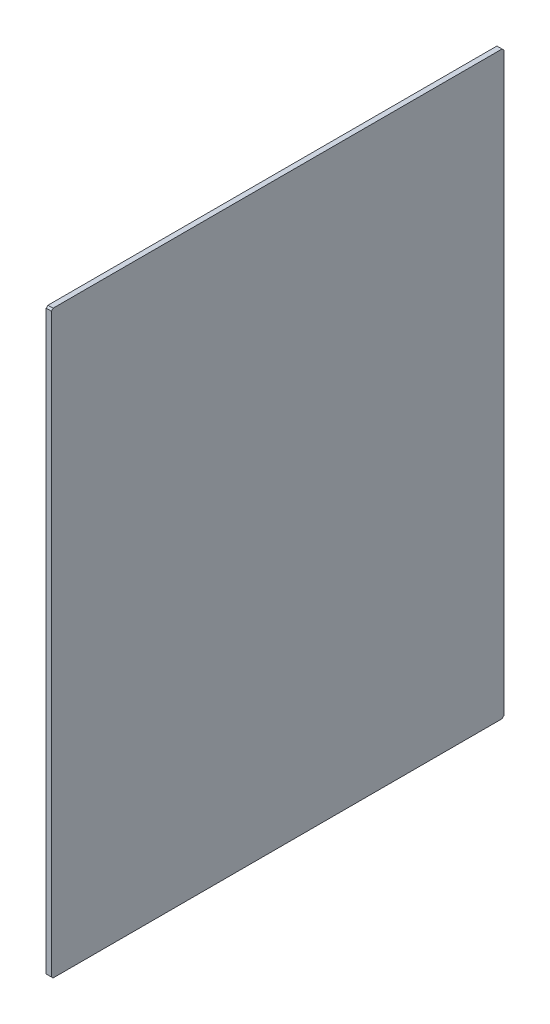
from build123d import *

# Parameters (mm, degrees)
SKETCH_1_W      = 528
SKETCH_1_H      = 677
EXTRUDE_1_DEPTH = 3
CHAMFER_1_SIZE  = 2


with BuildPart() as part:
    # 草图1 → 凸台-拉伸1 (new, symmetric)
    with BuildSketch(Plane(origin=(0, 0, 0), x_dir=(0, 0, -1), z_dir=(1, 0, 0))):
        Rectangle(SKETCH_1_W, SKETCH_1_H)
    extrude(amount=EXTRUDE_1_DEPTH, both=True)

    # 倒角1
    chamfer_1_edges = [part.edges().sort_by_distance(p)[0] for p in [
        (0, -338.5, -264),
        (0, -338.5, 264),
        (0, 338.5, 264),
        (0, 338.5, -264),
    ]]
    chamfer(chamfer_1_edges, length=CHAMFER_1_SIZE)


solid = part.part
